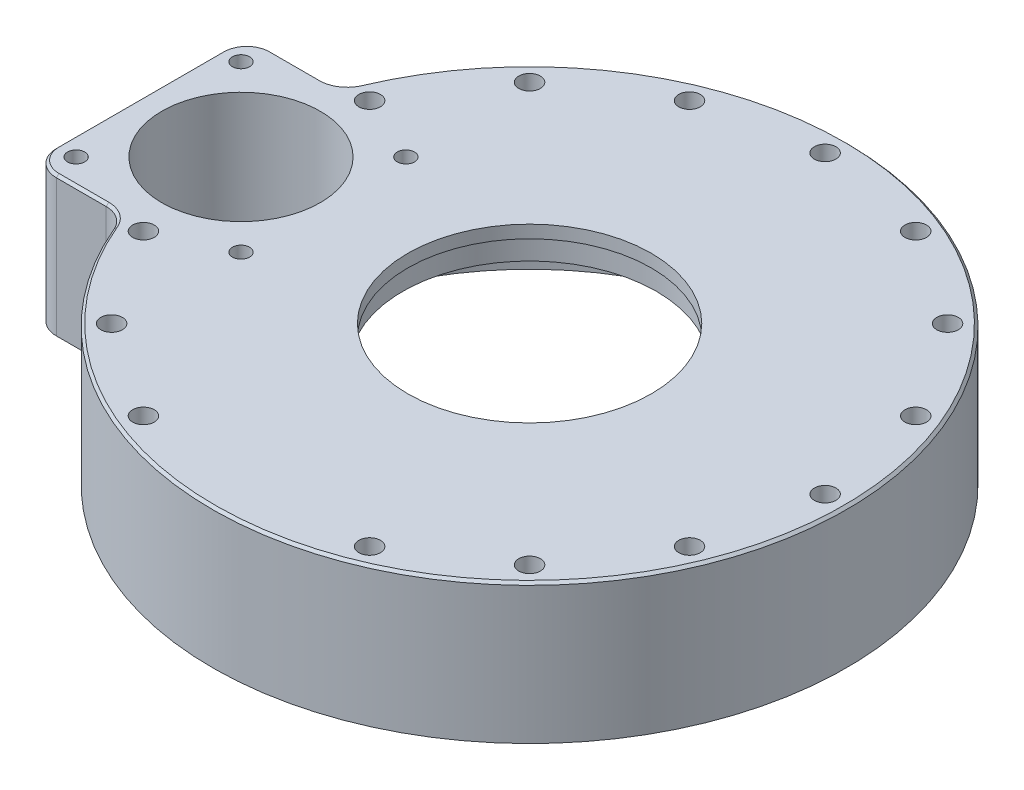
from build123d import *

# Parameters (mm, degrees)
SKETCH_3_W             = 50
SKETCH_3_H             = 85
EXTRUDE_1_DEPTH        = 55
SKETCH_5_R             = 31.25
CUT_EXTRUDE_1_DEPTH    = 45
HOLE_WIZARD_M8_1_D     = 6.8
HOLE_WIZARD_M8_1_DEPTH = 19.75
HOLE_WIZARD_M8_1_TIP   = 2.042926105
FILLET_1_R             = 10
HOLE_WIZARD_M10_1_D    = 8.5
CHAMFER_1_SIZE         = 1


with BuildPart() as part:
    # 草图2 → 旋转1 (revolve)
    with BuildSketch(Plane.XY, mode=Mode.PRIVATE) as revolve_1_sk:
        Polygon((104, 0), (104, 41), (50, 41), (50, 50), (48, 50), (48, 55), (125, 55), (125, 0), align=None)
    revolve(revolve_1_sk.sketch.rotate(Axis((0, 0, 0), (0, 1, 0)), 90), axis=Axis((0, 0, 0), (0, 1, 0)))

    # 草图3 → 凸台-拉伸1 (add, through all)
    with BuildSketch(Plane(origin=(0, 55, 0), x_dir=(1, 0, 0), z_dir=(0, 1, 0))):
        with Locations((-129, 0)):
            Rectangle(SKETCH_3_W, SKETCH_3_H)
    extrude(amount=-EXTRUDE_1_DEPTH)

    # 草图5 → 切除-拉伸1 (cut)
    with BuildSketch(Plane(origin=(0, 55, 0), x_dir=(1, 0, 0), z_dir=(0, 1, 0))):
        with Locations(Location((-113.75, 0, 0), (0, 0, 270))):
            Circle(SKETCH_5_R)
    extrude(amount=-CUT_EXTRUDE_1_DEPTH, mode=Mode.SUBTRACT)

    # M8 螺纹孔1
    with Locations(Plane(origin=(0, 55, 0), x_dir=(1, 0, 0), z_dir=(0, 1, 0))):
        with Locations((-146.25, 32.5), (-113.75, 0), (-81.25, 32.5), (-146.25, -32.5), (-81.25, -32.5)):
            Hole(HOLE_WIZARD_M8_1_D / 2, depth=HOLE_WIZARD_M8_1_DEPTH)
            with Locations((0, 0, -(HOLE_WIZARD_M8_1_DEPTH + HOLE_WIZARD_M8_1_TIP / 2))):  # 118° drill point
                Cone(0, HOLE_WIZARD_M8_1_D / 2, HOLE_WIZARD_M8_1_TIP, mode=Mode.SUBTRACT)

    # 圆角1
    fillet_1_edges = [part.edges().sort_by_distance(p)[0] for p in [
        (-117.553179455, 27.5, 42.5),
        (-117.553179455, 27.5, -42.5),
        (-154, 27.5, 42.5),
        (-154, 27.5, -42.5),
    ]]
    fillet(fillet_1_edges, radius=FILLET_1_R)

    # M10 螺纹孔1 (through all)
    with Locations(Plane(origin=(0, 0, 0), x_dir=(-1, 0, 0), z_dir=(0, -1, 0))):
        with Locations((-107.631965538, -44.582619871), (-107.631965538, 44.582619871), (-44.582619871, 107.631965538), (44.582619871, 107.631965538), (107.631965538, 44.582619871), (107.631965538, -44.582619871), (44.582619871, -107.631965538), (-44.582619871, -107.631965538), (0, 116.5), (-82.377940008, 82.377940008), (82.377940008, 82.377940008), (-82.377940008, -82.377940008), (82.377940008, -82.377940008), (-116.5, 0)):
            Hole(HOLE_WIZARD_M10_1_D / 2)

    # 倒角1
    chamfer_1_edges = [part.edges().sort_by_distance(p)[0] for p in [
        (-154, 55, 0),
        (125, 55, 0),
        (-134.186714819, 55, -42.5),
        (-134.186714819, 55, 42.5),
        (-151.071067812, 55, -39.571067812),
        (-151.071067812, 55, 39.571067812),
        (-118.845721654, 55, -44.166666667),
        (-118.845721654, 55, 44.166666667),
    ]]
    chamfer(chamfer_1_edges, length=CHAMFER_1_SIZE)


solid = part.part
